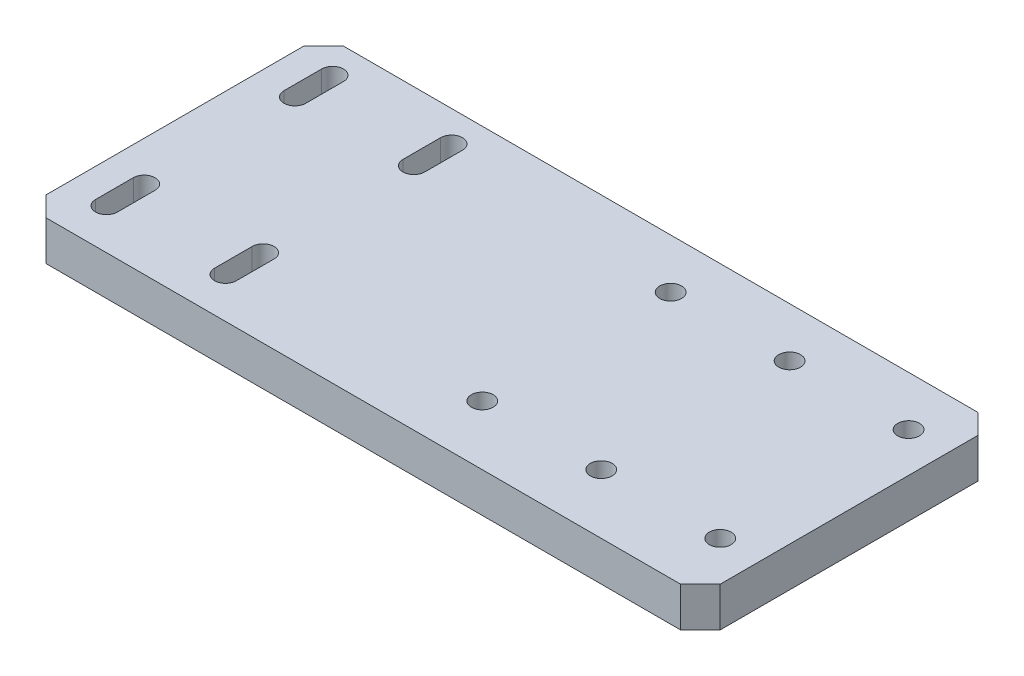
from build123d import *

# Parameters (mm, degrees)
SKETCH_1_W          = 170
SKETCH_1_H          = 75
EXTRUDE_1_DEPTH     = 10
CHAMFER_1_SIZE      = 5
SKETCH_2_R          = 2.75
CUT_EXTRUDE_1_DEPTH = 15


with BuildPart() as part:
    # 草图1 → 凸台-拉伸1 (new body)
    with BuildSketch(Plane(origin=(0, 0, 0), x_dir=(1, 0, 0), z_dir=(0, 1, 0))):
        Rectangle(SKETCH_1_W, SKETCH_1_H)
    extrude(amount=EXTRUDE_1_DEPTH)

    # 倒角1
    chamfer_1_edges = [part.edges().sort_by_distance(p)[0] for p in [
        (85, 5, 37.5),
        (-85, 5, 37.5),
        (-85, 5, -37.5),
        (85, 5, -37.5),
    ]]
    chamfer(chamfer_1_edges, length=CHAMFER_1_SIZE)

    # 草图2 → 切除-拉伸1 (cut)
    with BuildSketch(Plane(origin=(0, 10, 0), x_dir=(1, 0, 0), z_dir=(0, 1, 0))):
        with Locations(Location((15, 25, 0), (0, 0, 270))):
            Circle(SKETCH_2_R)
        with Locations(Location((45, 25, 0), (0, 0, 270))):
            Circle(SKETCH_2_R)
        with Locations(Location((75, 25, 0), (0, 0, 270))):
            Circle(SKETCH_2_R)
        with Locations(Location((15, -22.5, 0), (0, 0, 270))):
            Circle(SKETCH_2_R)
        with Locations(Location((45, -22.5, 0), (0, 0, 270))):
            Circle(SKETCH_2_R)
        with Locations(Location((75, -22.5, 0), (0, 0, 270))):
            Circle(SKETCH_2_R)
        with BuildLine():
            Line((-72.25, 29.75), (-72.25, 20.25))
            ThreePointArc((-72.25, 20.25), (-75, 17.5), (-77.75, 20.25))
            Line((-77.75, 20.25), (-77.75, 29.75))
            ThreePointArc((-77.75, 29.75), (-75, 32.5), (-72.25, 29.75))
        make_face()
        with BuildLine():
            Line((-42.25, 29.75), (-42.25, 20.25))
            ThreePointArc((-42.25, 20.25), (-45, 17.5), (-47.75, 20.25))
            Line((-47.75, 20.25), (-47.75, 29.75))
            ThreePointArc((-47.75, 29.75), (-45, 32.5), (-42.25, 29.75))
        make_face()
        with BuildLine():
            Line((-72.25, -17.75), (-72.25, -27.25))
            ThreePointArc((-72.25, -27.25), (-75, -30), (-77.75, -27.25))
            Line((-77.75, -27.25), (-77.75, -17.75))
            ThreePointArc((-77.75, -17.75), (-75, -15), (-72.25, -17.75))
        make_face()
        with BuildLine():
            Line((-42.25, -17.75), (-42.25, -27.25))
            ThreePointArc((-42.25, -27.25), (-45, -30), (-47.75, -27.25))
            Line((-47.75, -27.25), (-47.75, -17.75))
            ThreePointArc((-47.75, -17.75), (-45, -15), (-42.25, -17.75))
        make_face()
    extrude(amount=-CUT_EXTRUDE_1_DEPTH, mode=Mode.SUBTRACT)


solid = part.part
